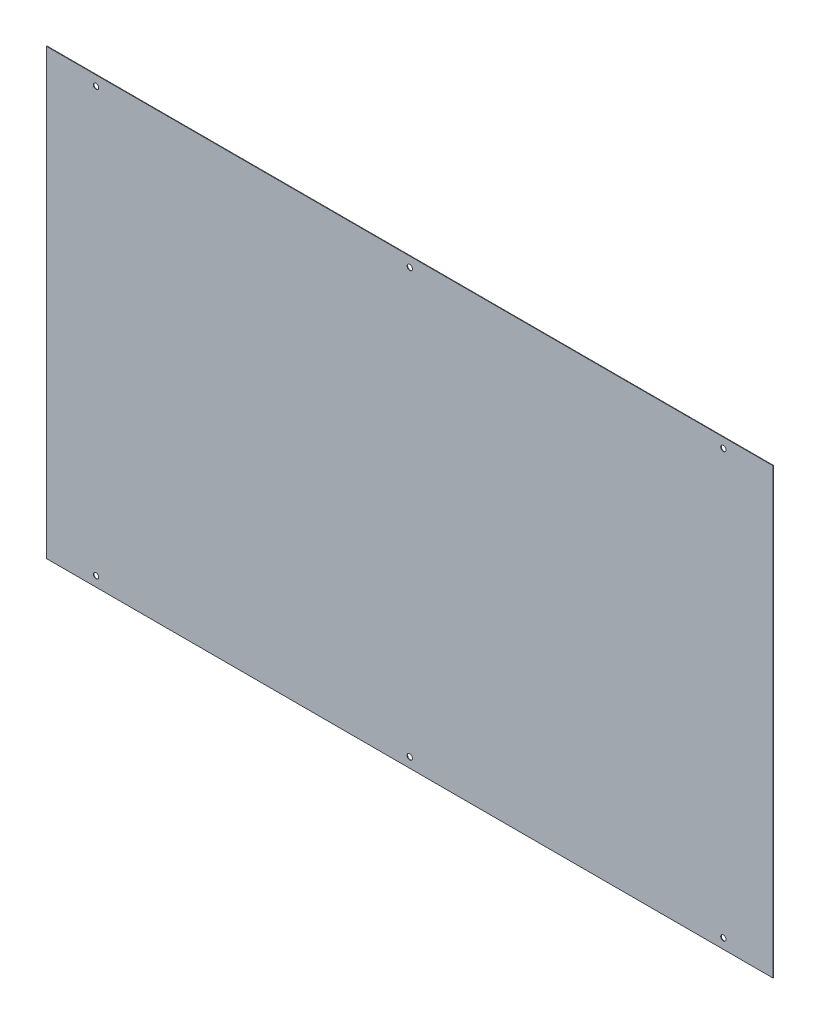
SolidWorks part; units mm, degrees
ref_plane "前视基准面" through (0, 0, 0) normal (0, 0, 1) x (1, 0, 0)
ref_plane "上视基准面" through (0, 0, 0) normal (0, 1, 0) x (1, 0, 0)
ref_plane "右视基准面" through (0, 0, 0) normal (1, 0, 0) x (0, 0, -1)
sketch "草图1" plane through (0, 0, 0) normal (0, 0, 1) x (1, 0, 0)
  line L1 (-550, 336) -> (550, 336)
  line L2 (-550, 336) -> (-550, -336)
  line L3 (-550, -336) -> (550, -336)
  line L4 (550, 336) -> (550, -336)
  line L5 (-550, 336) -> (550, -336) construction
  line L6 (-550, -336) -> (550, 336) construction
  point P0 (0, 0)
  dimension "D1" = 672
  dimension "D2" = 1100
extrude "凸台-拉伸1" add sketch "草图1" along normal blind 0.8
sketch "草图2" plane through (0, 0, 0) normal (0, 0, -1) x (-1, 0, 0)
  line L0 (550, 321) -> (-554.8475, 321) construction
  line L1 (550, 336) -> (550, -336) construction
  line L2 (-550, 336) -> (550, 336) construction
  line L3 (0, 0) -> (0, 491.7025) construction
  line L4 (0, 0) -> (-823.3143, 0) construction
  circle A0 centre (0, 321) radius 4
  circle A1 centre (475, 321) radius 4
  circle A2 centre (-475, 321) radius 4
  circle A3 centre (-475, -321) radius 4
  circle A4 centre (475, -321) radius 4
  circle A5 centre (0, -321) radius 4
  dimension "D2" = 8
  dimension "D1" = 15
extrude "切除-拉伸1" cut sketch "草图2" against normal blind 0.8
